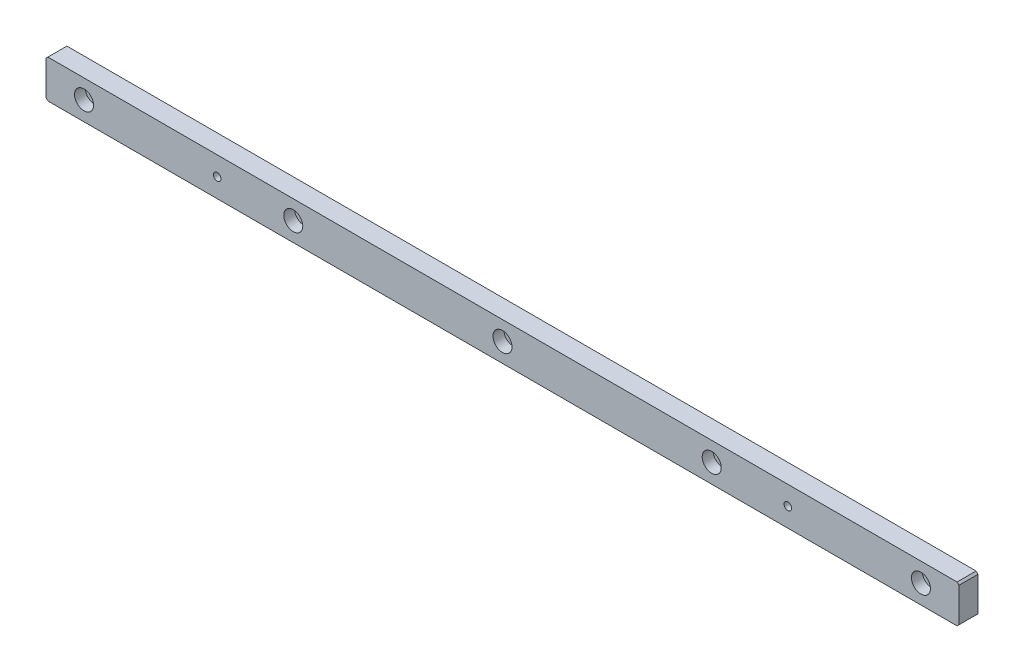
SolidWorks part; units mm, degrees
ref_plane "Front Plane" through (0, 0, 0) normal (0, 0, 1) x (1, 0, 0)
ref_plane "Top Plane" through (0, 0, 0) normal (0, 1, 0) x (1, 0, 0)
ref_plane "Right Plane" through (0, 0, 0) normal (1, 0, 0) x (0, 0, -1)
sketch "Sketch1" plane through (0, 0, 0) normal (0, 0, 1) x (1, 0, 0)
  line L1 (-240, 10) -> (240, 10)
  line L2 (-240, 10) -> (-240, -10)
  line L3 (-240, -10) -> (240, -10)
  line L4 (240, 10) -> (240, -10)
  line L5 (-240, 10) -> (240, -10) construction
  line L6 (-240, -10) -> (240, 10) construction
  point P0 (0, 0)
  dimension "D1" = 20
  dimension "D2" = 480
extrude "Boss-Extrude1" add sketch "Sketch1" along normal blind 10
hole_wizard "Hole size per socket head cap screw type1" positions "Sketch3" profile "Sketch2" counterbore size "M5" standard "GB" end condition through all
sketch "Sketch3" plane through (0, 0, 10) normal (0, 0, 1) x (1, 0, 0)
  point P1 (0, 0)
  point P4 (-110, 0)
  point P6 (110, 0)
  point P8 (220, 0)
  point P14 (-220, 0)
  dimension "D1" = 110
  dimension "D2" = 110
  dimension "D3" = 110
  dimension "D4" = 110
sketch "Sketch2" plane through (0, 0, 10) normal (1, 0, 0) x (0, -1, 0)
  line L0 (0, 0) -> (0, 10)
  line L1 (0, 10) -> (2.75, 10)
  line L3 (2.75, 10) -> (2.75, 5.7)
  line L4 (2.75, 5.7) -> (5, 5.7)
  line L5 (5, 5.7) -> (5, 0)
  line L7 (5, 0) -> (0, 0)
  line L11 (0, -6.35) -> (0, 107.95) construction
  dimension "通孔孔直径" = 5.5
  dimension "通孔孔深度" = 10
  dimension "柱形沉头孔直径" = 10
  dimension "柱形沉头孔深度" = 5.7
chamfer "Chamfer1" distance 1 angle 45 4 edges at (240, -10, 5) (240, 10, 5) (-240, 10, 5) (-240, -10, 5)
hole_wizard "Ø4.0 (4) Diameter Hole1" positions "Sketch5" profile "Sketch4" hole size "Ø4.0" standard "GB"
sketch "Sketch5" plane through (0, 0, 10) normal (0, 0, 1) x (1, 0, 0)
  line L0 (0, 10) -> (0, -26.4508) construction
  line L1 (239, 10) -> (-239, 10) construction
  point P0 (-150, 0)
  point P1 (150, 0)
  dimension "D1" = 300
sketch "Sketch4" plane through (-150, 0, 10) normal (1, 0, 0) x (0, -1, 0)
  line L0 (0, 0) -> (0, 13.2017)
  line L1 (0, 13.2017) -> (2, 12)
  line L2 (2, 12) -> (2, 0)
  line L5 (2, 0) -> (0, 0)
  line L10 (0, 13.2017) -> (-2, 12) construction
  line L11 (0, -6.35) -> (0, 107.95) construction
  dimension "孔直径" = 4
  dimension "孔深度" = 12
  dimension "导头角度" = 118
